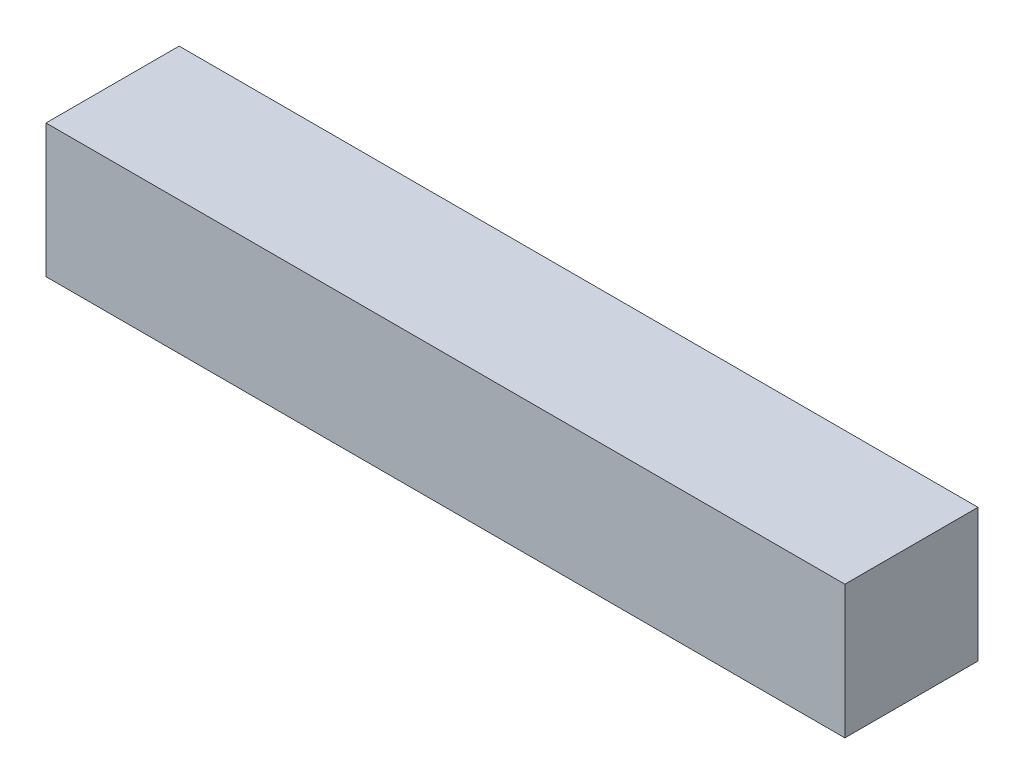
from build123d import *

# Parameters (mm, degrees)
SKETCH_1_W      = 10
SKETCH_1_H      = 10
EXTRUDE_1_DEPTH = 60


with BuildPart() as part:
    # 草图1 → 凸台-拉伸1 (new body)
    with BuildSketch(Plane(origin=(0, 0, 0), x_dir=(0, 0, -1), z_dir=(1, 0, 0))):
        Rectangle(SKETCH_1_W, SKETCH_1_H)
    extrude(amount=EXTRUDE_1_DEPTH)


solid = part.part
